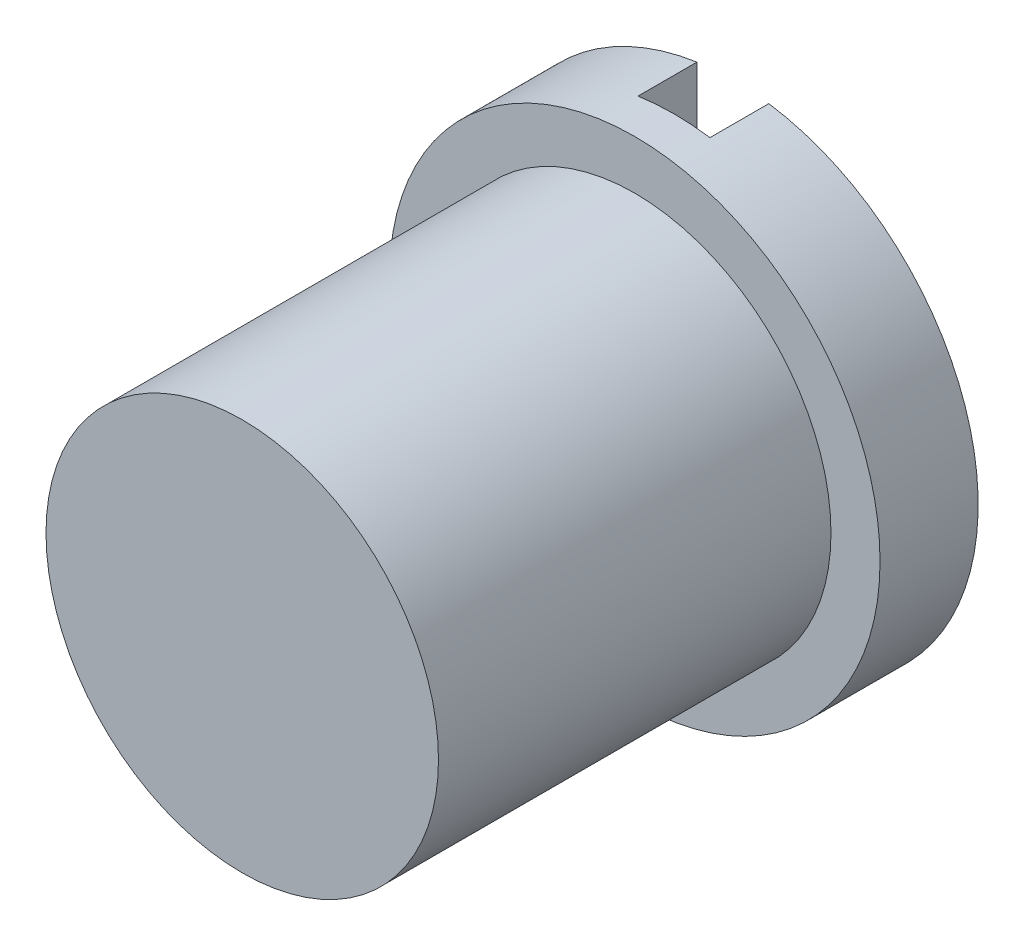
from build123d import *

# Parameters (mm, degrees)
SKETCH1_R           = 12.5
BOSS_EXTRUDE1_DEPTH = 5
SKETCH2_R           = 10
BOSS_EXTRUDE2_DEPTH = 20
CUT_EXTRUDE2_DEPTH  = 3


with BuildPart() as part:
    # Sketch1 → Boss-Extrude1 (new body)
    with BuildSketch(Plane.XY):
        Circle(SKETCH1_R)
    extrude(amount=BOSS_EXTRUDE1_DEPTH)

    # Sketch2 → Boss-Extrude2 (add)
    with BuildSketch(Plane.XY.offset(5)):
        Circle(SKETCH2_R)
    extrude(amount=BOSS_EXTRUDE2_DEPTH)

    # Sketch3 → Cut-Extrude2 (cut)
    with BuildSketch(Plane(origin=(0, 0, 0), x_dir=(-1, 0, 0), z_dir=(0, 0, -1))):
        with BuildLine():
            Line((1.83229916, 12.364977953), (1.83229916, -12.364977953))
            ThreePointArc((1.83229916, -12.364977953), (0, -12.5), (-1.83229916, -12.364977953))
            Line((-1.83229916, -12.364977953), (-1.83229916, 12.364977953))
            ThreePointArc((-1.83229916, 12.364977953), (0, 12.5), (1.83229916, 12.364977953))
        make_face()
    extrude(amount=-CUT_EXTRUDE2_DEPTH, mode=Mode.SUBTRACT)


solid = part.part
